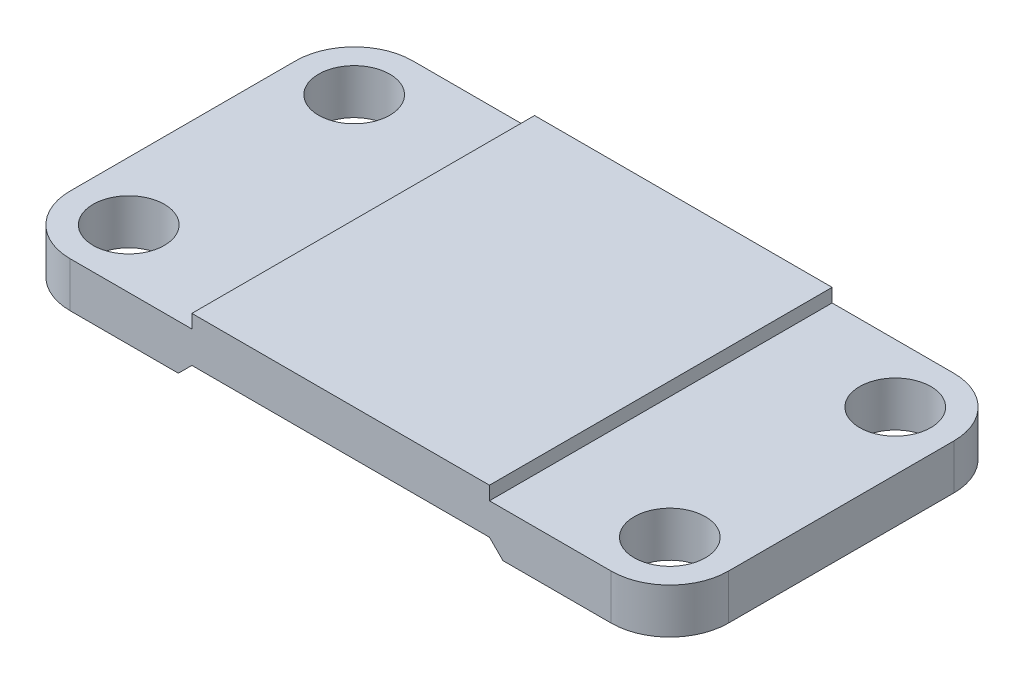
SolidWorks part; units mm, degrees
ref_plane "Front Plane" through (0, 0, 0) normal (0, 0, 1) x (1, 0, 0)
ref_plane "Top Plane" through (0, 0, 0) normal (0, 1, 0) x (1, 0, 0)
ref_plane "Right Plane" through (0, 0, 0) normal (1, 0, 0) x (0, 0, -1)
sketch "Sketch1" plane through (0, 0, 0) normal (0, 1, 0) x (1, 0, 0)
  line L1 (1524, 965.2) -> (-1524, 965.2)
  line L2 (1854.2, 635) -> (1854.2, -635)
  line L3 (1524, -965.2) -> (-1524, -965.2)
  line L4 (-1854.2, 635) -> (-1854.2, -635)
  line L5 (1854.2, 965.2) -> (-1854.2, -965.2) construction
  line L6 (1854.2, -965.2) -> (-1854.2, 965.2) construction
  arc A0 (-1524, 965.2) -> (-1854.2, 635) centre (-1524, 635) ccw
  arc A1 (1854.2, -635) -> (1524, -965.2) centre (1524, -635) cw
  arc A2 (1524, 965.2) -> (1854.2, 635) centre (1524, 635) cw
  arc A3 (-1524, -965.2) -> (-1854.2, -635) centre (-1524, -635) cw
  circle A4 centre (-1524, 635) radius 200.7207
  circle A5 centre (1524, 635) radius 200.7207
  circle A6 centre (1524, -635) radius 200.7207
  circle A7 centre (-1524, -635) radius 200.7207
  point P0 (0, 0)
  dimension "D1" = 330.2
extrude "Boss-Extrude1" add sketch "Sketch1" along normal blind 330.2
sketch "Sketch3" plane through (0, 330.2, 0) normal (0, 1, 0) x (1, 0, 0)
  line L0 (-838.2, 965.2) -> (-838.2, -965.2)
  line L1 (1524, 965.2) -> (-1524, 965.2) construction
  line L2 (-1524, -965.2) -> (1524, -965.2) construction
  line L3 (838.2, 965.2) -> (838.2, -965.2)
  line L4 (-1854.2, 635) -> (-1854.2, -635) construction
  line L5 (838.2, -965.2) -> (-838.2, -965.2)
  line L6 (-838.2, 965.2) -> (838.2, 965.2)
  dimension "D1" = 1676.4
  dimension "D2" = 1016
extrude "Boss-Extrude4" add sketch "Sketch3" along normal blind 76.2
sketch "Sketch5" plane through (0, 0, 0) normal (0, -1, 0) x (1, 0, 0)
  line L4 (-1524, -965.2) -> (1524, -965.2)
  line L5 (1854.2, -635) -> (1854.2, 635)
  line L6 (1524, 965.2) -> (-1524, 965.2)
  line L7 (-1854.2, 635) -> (-1854.2, -635)
  line L8 (-1524, -965.2) -> (1524, -965.2)
  line L9 (1854.2, -635) -> (1854.2, 635)
  line L10 (1524, 965.2) -> (-1524, 965.2)
  line L11 (-1854.2, 635) -> (-1854.2, -635)
  arc A4 (-1854.2, -635) -> (-1524, -965.2) centre (-1524, -635) ccw
  arc A5 (1524, -965.2) -> (1854.2, -635) centre (1524, -635) ccw
  arc A6 (1854.2, 635) -> (1524, 965.2) centre (1524, 635) ccw
  arc A7 (-1524, 965.2) -> (-1854.2, 635) centre (-1524, 635) ccw
  arc A8 (-1854.2, -635) -> (-1524, -965.2) centre (-1524, -635) ccw
  arc A9 (1524, -965.2) -> (1854.2, -635) centre (1524, -635) ccw
  arc A10 (1854.2, 635) -> (1524, 965.2) centre (1524, 635) ccw
  arc A11 (-1524, 965.2) -> (-1854.2, 635) centre (-1524, 635) ccw
  dimension "D1" = 0
extrude "Cut-Extrude2" cut sketch "Sketch5" against normal blind 76.2
sketch "Sketch6" plane through (0, 0, 965.2) normal (0, 0, 1) x (1, 0, 0)
  line L0 (914.4, 76.2) -> (-914.4, 76.2)
  line L1 (1524, 76.2) -> (-1524, 76.2) construction
  line L3 (-838.2, 330.2) -> (-838.2, 152.4)
  line L4 (838.2, 330.2) -> (838.2, 152.4)
  line L5 (838.2, 152.4) -> (-838.2, 152.4)
  line L7 (-914.4, 76.2) -> (-838.2, 152.4)
  line L8 (838.2, 152.4) -> (914.4, 76.2)
  line M4 (-1524, 76.2) -> (1524, 76.2)
extrude "Cut-Extrude6" cut sketch "Sketch6" against normal through all contours L8 L5 L7 M4
